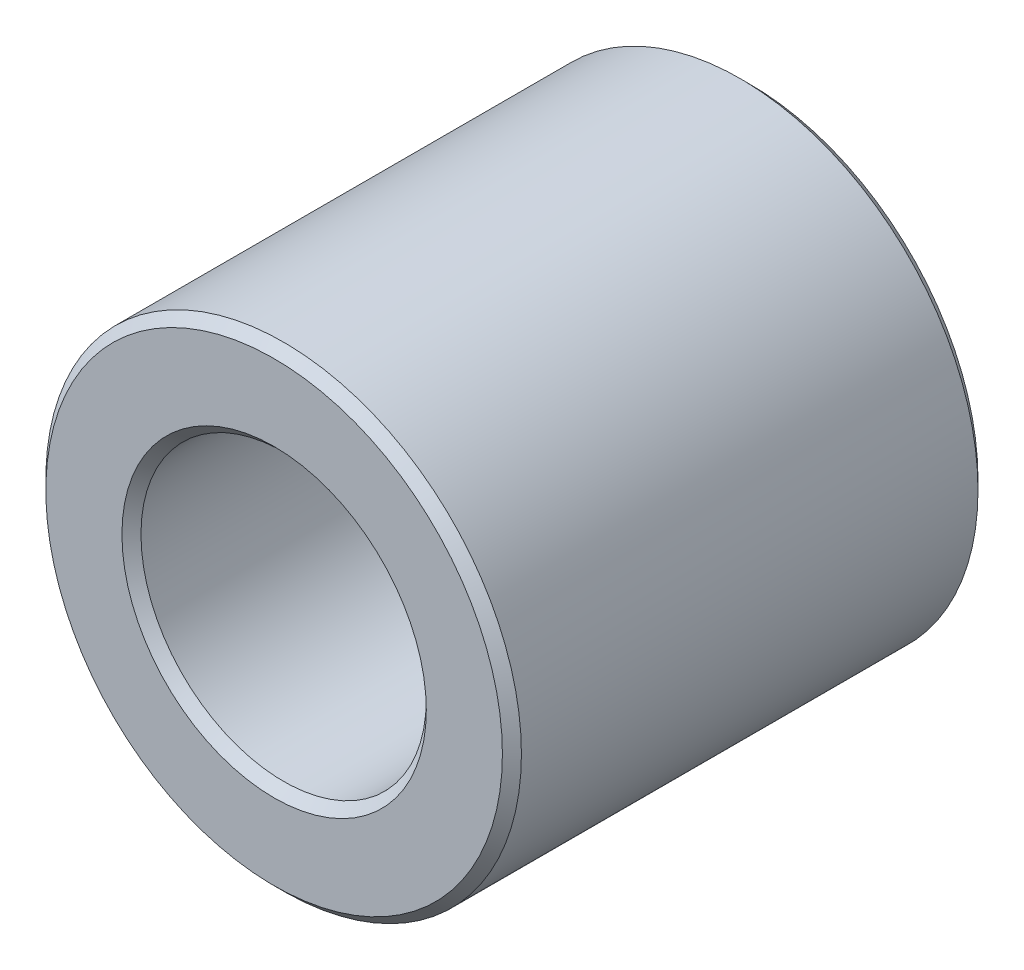
from build123d import *

# Parameters (mm, degrees)
SKETCH1_R           = 25
SKETCH1_R_2         = 15
BOSS_EXTRUDE1_DEPTH = 50
CHAMFER1_SIZE       = 1


with BuildPart() as part:
    # Sketch1 → Boss-Extrude1 (new body)
    with BuildSketch(Plane.XY):
        Circle(SKETCH1_R)
        Circle(SKETCH1_R_2, mode=Mode.SUBTRACT)
    extrude(amount=BOSS_EXTRUDE1_DEPTH)

    # Chamfer1
    chamfer1_edges = [part.edges().sort_by_distance(p)[0] for p in [
        (-25, 0, 0),
        (-25, 0, 50),
        (-15, 0, 0),
        (-15, 0, 50),
    ]]
    chamfer(chamfer1_edges, length=CHAMFER1_SIZE)


solid = part.part
